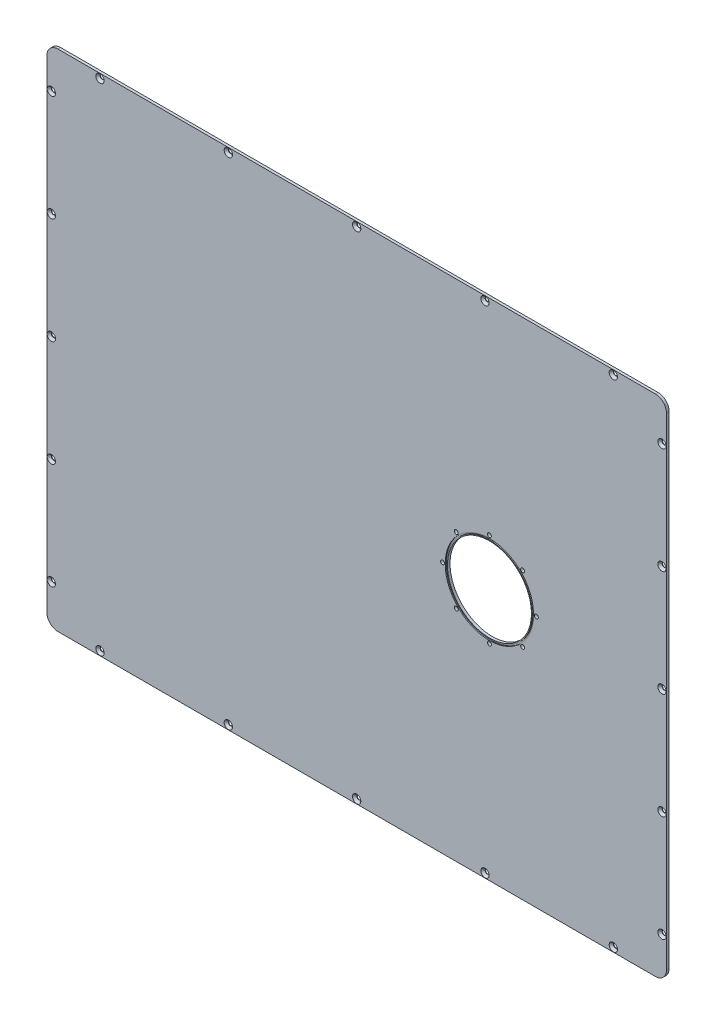
from build123d import *

# Parameters (mm, degrees)
EXTRUDE_1_DEPTH              = 3
HOLE_WIZARD_M4_1_D           = 4.5
HOLE_WIZARD_M4_1_DEPTH       = 10.1
HOLE_WIZARD_M4_1_CSINK_D     = 9.4
HOLE_WIZARD_M4_1_CSINK_ANGLE = 90
HOLE_WIZARD_M4_1_TIP         = 1.351936393
SKETCH_4_R                   = 47.5
CUT_EXTRUDE_1_DEPTH          = 12
SKETCH_5_R                   = 50
SKETCH_5_R_2                 = 48.5
CUT_EXTRUDE_2_DEPTH          = 1.2
SKETCH_6_R                   = 2.25
CUT_EXTRUDE_3_DEPTH          = 10


with BuildPart() as part:
    # 草图1 → 凸台-拉伸1 (new body)
    with BuildSketch(Plane.XY):
        with BuildLine():
            Line((227.012333385, 39.0187092), (227.012333385, 584.0187092))
            ThreePointArc((227.012333385, 584.0187092), (223.35116815, 592.857543965), (214.512333385, 596.5187092))
            Line((214.512333385, 596.5187092), (-460.487666615, 596.5187092))
            ThreePointArc((-460.487666615, 596.5187092), (-469.326501379, 592.857543965), (-472.987666615, 584.0187092))
            Line((-472.987666615, 584.0187092), (-472.987666615, 39.0187092))
            ThreePointArc((-472.987666615, 39.0187092), (-469.326501379, 30.179874435), (-460.487666615, 26.5187092))
            Line((-460.487666615, 26.5187092), (214.512333385, 26.5187092))
            ThreePointArc((214.512333385, 26.5187092), (223.35116815, 30.179874435), (227.012333385, 39.0187092))
        make_face()
    extrude(amount=EXTRUDE_1_DEPTH)

    # M4 锥坑平头螺钉的锥形沉头孔1
    with Locations(Plane.XY.offset(3)):
        with Locations((222.012333385, 71.5187092), (222.012333385, 191.5187092), (222.012333385, 311.5187092), (222.012333385, 431.5187092), (222.012333385, 551.5187092), (167.012333385, 591.5187092), (22.012333385, 591.5187092), (-122.987666615, 591.5187092), (-267.987666615, 591.5187092), (-412.987666615, 591.5187092), (-467.987666615, 551.5187092), (-467.987666615, 431.5187092), (-467.987666615, 311.5187092), (-467.987666615, 191.5187092), (-467.987666615, 71.5187092), (-412.987666615, 31.5187092), (-267.987666615, 31.5187092), (-122.987666615, 31.5187092), (22.012333385, 31.5187092), (167.012333385, 31.5187092)):
            CounterSinkHole(HOLE_WIZARD_M4_1_D / 2, HOLE_WIZARD_M4_1_CSINK_D / 2, depth=HOLE_WIZARD_M4_1_DEPTH, counter_sink_angle=HOLE_WIZARD_M4_1_CSINK_ANGLE)
            with Locations((0, 0, -(HOLE_WIZARD_M4_1_DEPTH + HOLE_WIZARD_M4_1_TIP / 2))):  # 118° drill point
                Cone(0, HOLE_WIZARD_M4_1_D / 2, HOLE_WIZARD_M4_1_TIP, mode=Mode.SUBTRACT)

    # 草图4 → 切除-拉伸1 (cut)
    with BuildSketch(Plane.XY.offset(3)):
        with Locations((27.012333385, 311.5187092)):
            Circle(SKETCH_4_R)
    extrude(amount=-CUT_EXTRUDE_1_DEPTH, mode=Mode.SUBTRACT)

    # 草图5 → 切除-拉伸2 (cut)
    with BuildSketch(Plane.XY.offset(3)):
        with Locations((27.012333385, 311.5187092)):
            Circle(SKETCH_5_R)
        with Locations((27.012333385, 311.5187092)):
            Circle(SKETCH_5_R_2, mode=Mode.SUBTRACT)
    extrude(amount=-CUT_EXTRUDE_2_DEPTH, mode=Mode.SUBTRACT)

    # 草图6 → 切除-拉伸3 (cut)
    with BuildSketch(Plane.XY.offset(3)):
        with Locations((27.012333385, 258.5187092)):
            Circle(SKETCH_6_R)
        with Locations((-10.464326017, 274.042049797)):
            Circle(SKETCH_6_R)
        with Locations((-25.987666615, 311.5187092)):
            Circle(SKETCH_6_R)
        with Locations((-10.464326017, 348.995368603)):
            Circle(SKETCH_6_R)
        with Locations((27.012333385, 364.5187092)):
            Circle(SKETCH_6_R)
        with Locations((64.488992788, 348.995368603)):
            Circle(SKETCH_6_R)
        with Locations((80.012333385, 311.5187092)):
            Circle(SKETCH_6_R)
        with Locations((64.488992788, 274.042049797)):
            Circle(SKETCH_6_R)
    extrude(amount=-CUT_EXTRUDE_3_DEPTH, mode=Mode.SUBTRACT)


solid = part.part
